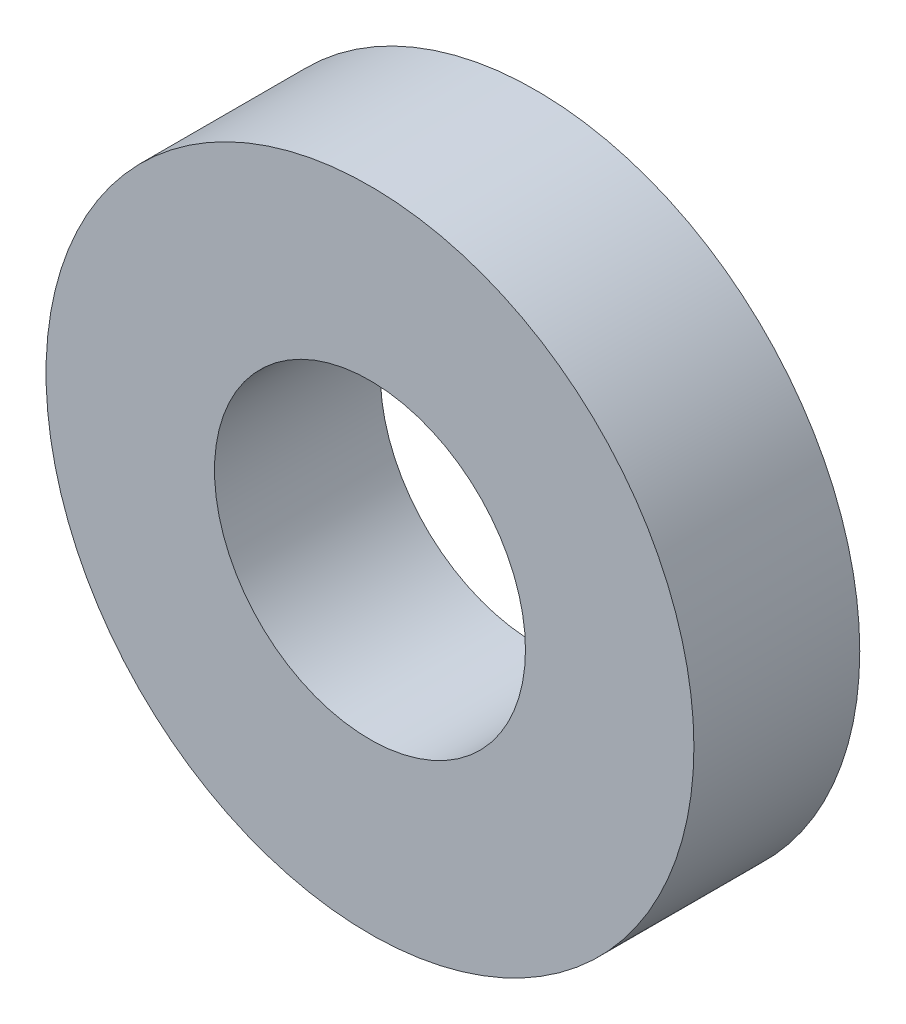
from build123d import *

# Parameters (mm, degrees)
SKETCH_1_R      = 62.5
SKETCH_1_R_2    = 30
EXTRUDE_1_DEPTH = 16


with BuildPart() as part:
    # 草图1 → 凸台-拉伸1 (new, symmetric)
    with BuildSketch(Plane.XY):
        Circle(SKETCH_1_R)
        Circle(SKETCH_1_R_2, mode=Mode.SUBTRACT)
    extrude(amount=EXTRUDE_1_DEPTH, both=True)


solid = part.part
